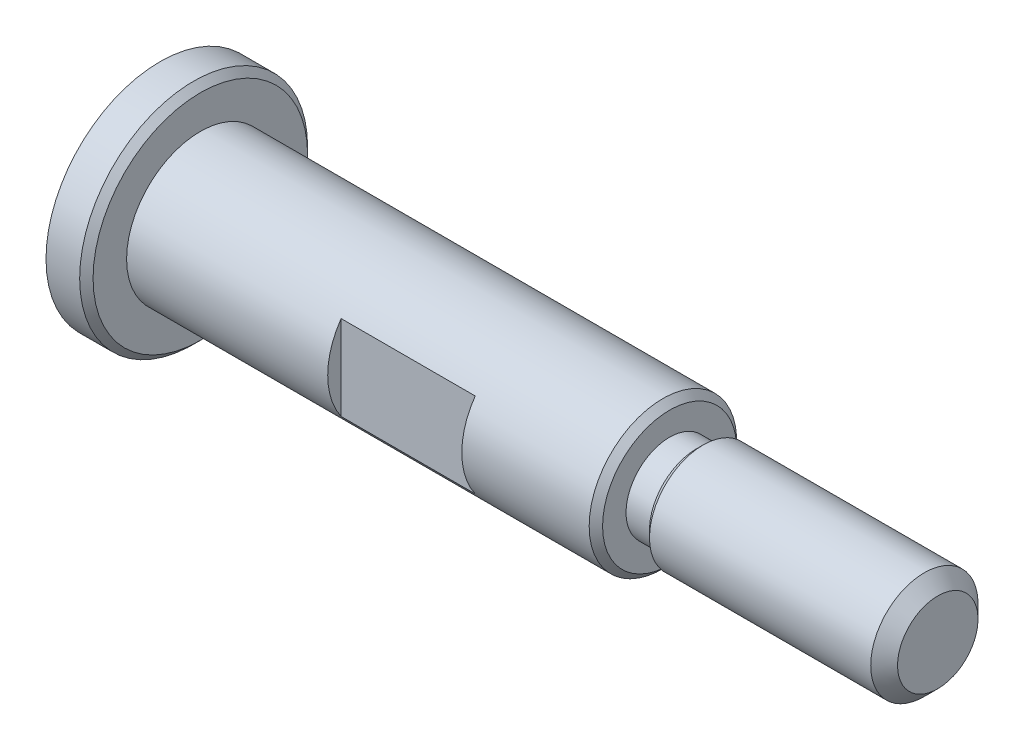
SolidWorks part; units mm, degrees
ref_plane "Front Plane" through (0, 0, 0) normal (0, 0, 1) x (1, 0, 0)
ref_plane "Top Plane" through (0, 0, 0) normal (0, 1, 0) x (1, 0, 0)
ref_plane "Right Plane" through (0, 0, 0) normal (1, 0, 0) x (0, 0, -1)
sketch "Sketch1" plane through (0, 0, 0) normal (0, 0, 1) x (1, 0, 0)
  line L0 (0, 0) -> (156.0731, 0) construction
  line L1 (59.5, 3) -> (58.5, 4)
  line L3 (1.4894, 8.5) -> (4.5, 8.5)
  line L4 (4.5, 5.5) -> (4.5, 8.5)
  line L8 (4.5, 5.5) -> (39.5, 5.5)
  line L9 (39.5, 4) -> (39.5, 5.5)
  line L10 (0, 0) -> (59.5, 0)
  line L12 (39.5, 4) -> (58.5, 4)
  line L13 (59.5, 0) -> (59.5, 3)
  arc A0 (1.4894, 8.5) -> (0, 0) centre (25, 0) ccw
  point P9 (59.5, 4)
  dimension "D7" = 50
  dimension "D1" = 17
  dimension "D2" = 11
  dimension "D3" = 8
  dimension "D4" = 4.5
  dimension "D5" = 35
  dimension "D6" = 20
revolve "Revolve1" add sketch "Sketch1" angle 360 about L0
cosmetic thread "Cosmetic Thread1" parameters "D2"=6.917
sketch "Sketch2" plane through (0, 0, 0) normal (0, 1, 0) x (1, 0, 0)
  line L0 (39.5, 5.5) -> (4.5, 5.5) construction
  line L1 (19.5, 5.5) -> (29.5, 5.5)
  line L2 (19.5, 5.5) -> (19.5, 4.5)
  line L3 (19.5, 4.5) -> (29.5, 4.5)
  line L4 (29.5, 5.5) -> (29.5, 4.5)
  line L5 (4.5, -8.5) -> (4.5, 8.5) construction
  dimension "D1" = 1
  dimension "D2" = 10
  dimension "D3" = 15
extrude "Cut-Extrude2" cut sketch "Sketch2" against normal mid plane 10
mirror "Mirror1" about plane through (0, 0, 0) normal (0, 0, 1) of "Cut-Extrude2"
chamfer "Chamfer1" distance 0.5 angle 45 2 edges at (39.5, 0, 5.5) (4.5, 0, 8.5)
sketch "Sketch3" plane through (0, 0, 0) normal (0, 1, 0) x (1, 0, 0)
  line L1 (39.5, 4) -> (41.5, 4)
  line L2 (39.5, 4) -> (39.5, 3.25)
  line L3 (39.5, 3.25) -> (41.5, 3.25)
  line L4 (41.5, 4) -> (41.5, 3.25)
  dimension "D1" = 2
  dimension "D2" = 0.75
ref_axis "Axis1" through (58.5, 0, 0) along (-1, 0, 0)
revolve "Cut-Revolve1" cut sketch "Sketch3" angle 360 about axis through (58.5, 0, 0) along (-1, 0, 0)
chamfer "Chamfer2" distance 0.5 angle 45 1 edges at (41.5, 0, -4)
